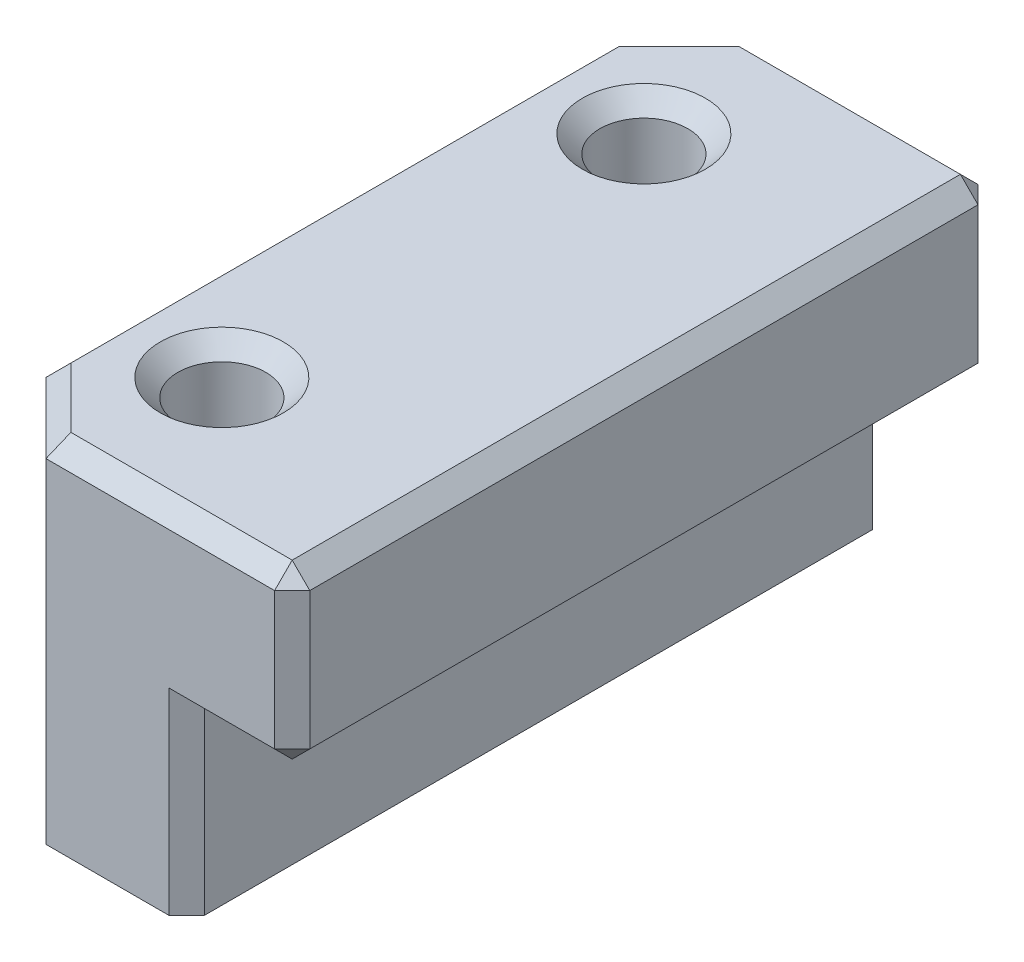
from build123d import *

# Parameters (mm, degrees)
EXTRUDE_1_DEPTH    = 20
HOLE_WIZARD_M3_1_D = 2.5
CHAMFER_1_SIZE     = 2
CHAMFER_2_SIZE     = 0.5


with BuildPart() as part:
    # 草图1 → 凸台-拉伸1 (new body)
    with BuildSketch(Plane.XY):
        Polygon((0, 0), (6, 0), (6, 5.1), (9, 5.1), (9, 10), (0, 10), align=None)
    extrude(amount=EXTRUDE_1_DEPTH)

    # M3 螺纹孔1 (through all)
    with Locations(Plane(origin=(0, 10, 0), x_dir=(1, 0, 0), z_dir=(0, 1, 0))):
        with Locations((3, -16), (3, -4)):
            Hole(HOLE_WIZARD_M3_1_D / 2)

    # 倒角1
    chamfer_1_edges = [part.edges().sort_by_distance(p)[0] for p in [
        (0, 5, 20),
        (0, 5, 0),
    ]]
    chamfer(chamfer_1_edges, length=CHAMFER_1_SIZE)

    # 倒角2
    chamfer_2_edges = [part.edges().sort_by_distance(p)[0] for p in [
        (6, 2.55, 20),
        (9, 10, 10),
        (9, 5.1, 10),
        (7.5, 5.1, 20),
        (0, 10, 10),
        (1, 10, 19),
        (1, 10, 1),
        (9, 7.55, 20),
        (5.5, 10, 20),
        (4.25, 10, 4),
        (4.25, 10, 16),
        (5.5, 10, 0),
        (9, 7.55, 0),
        (7.5, 5.1, 0),
        (6, 2.55, 0),
    ]]
    chamfer(chamfer_2_edges, length=CHAMFER_2_SIZE)


solid = part.part
